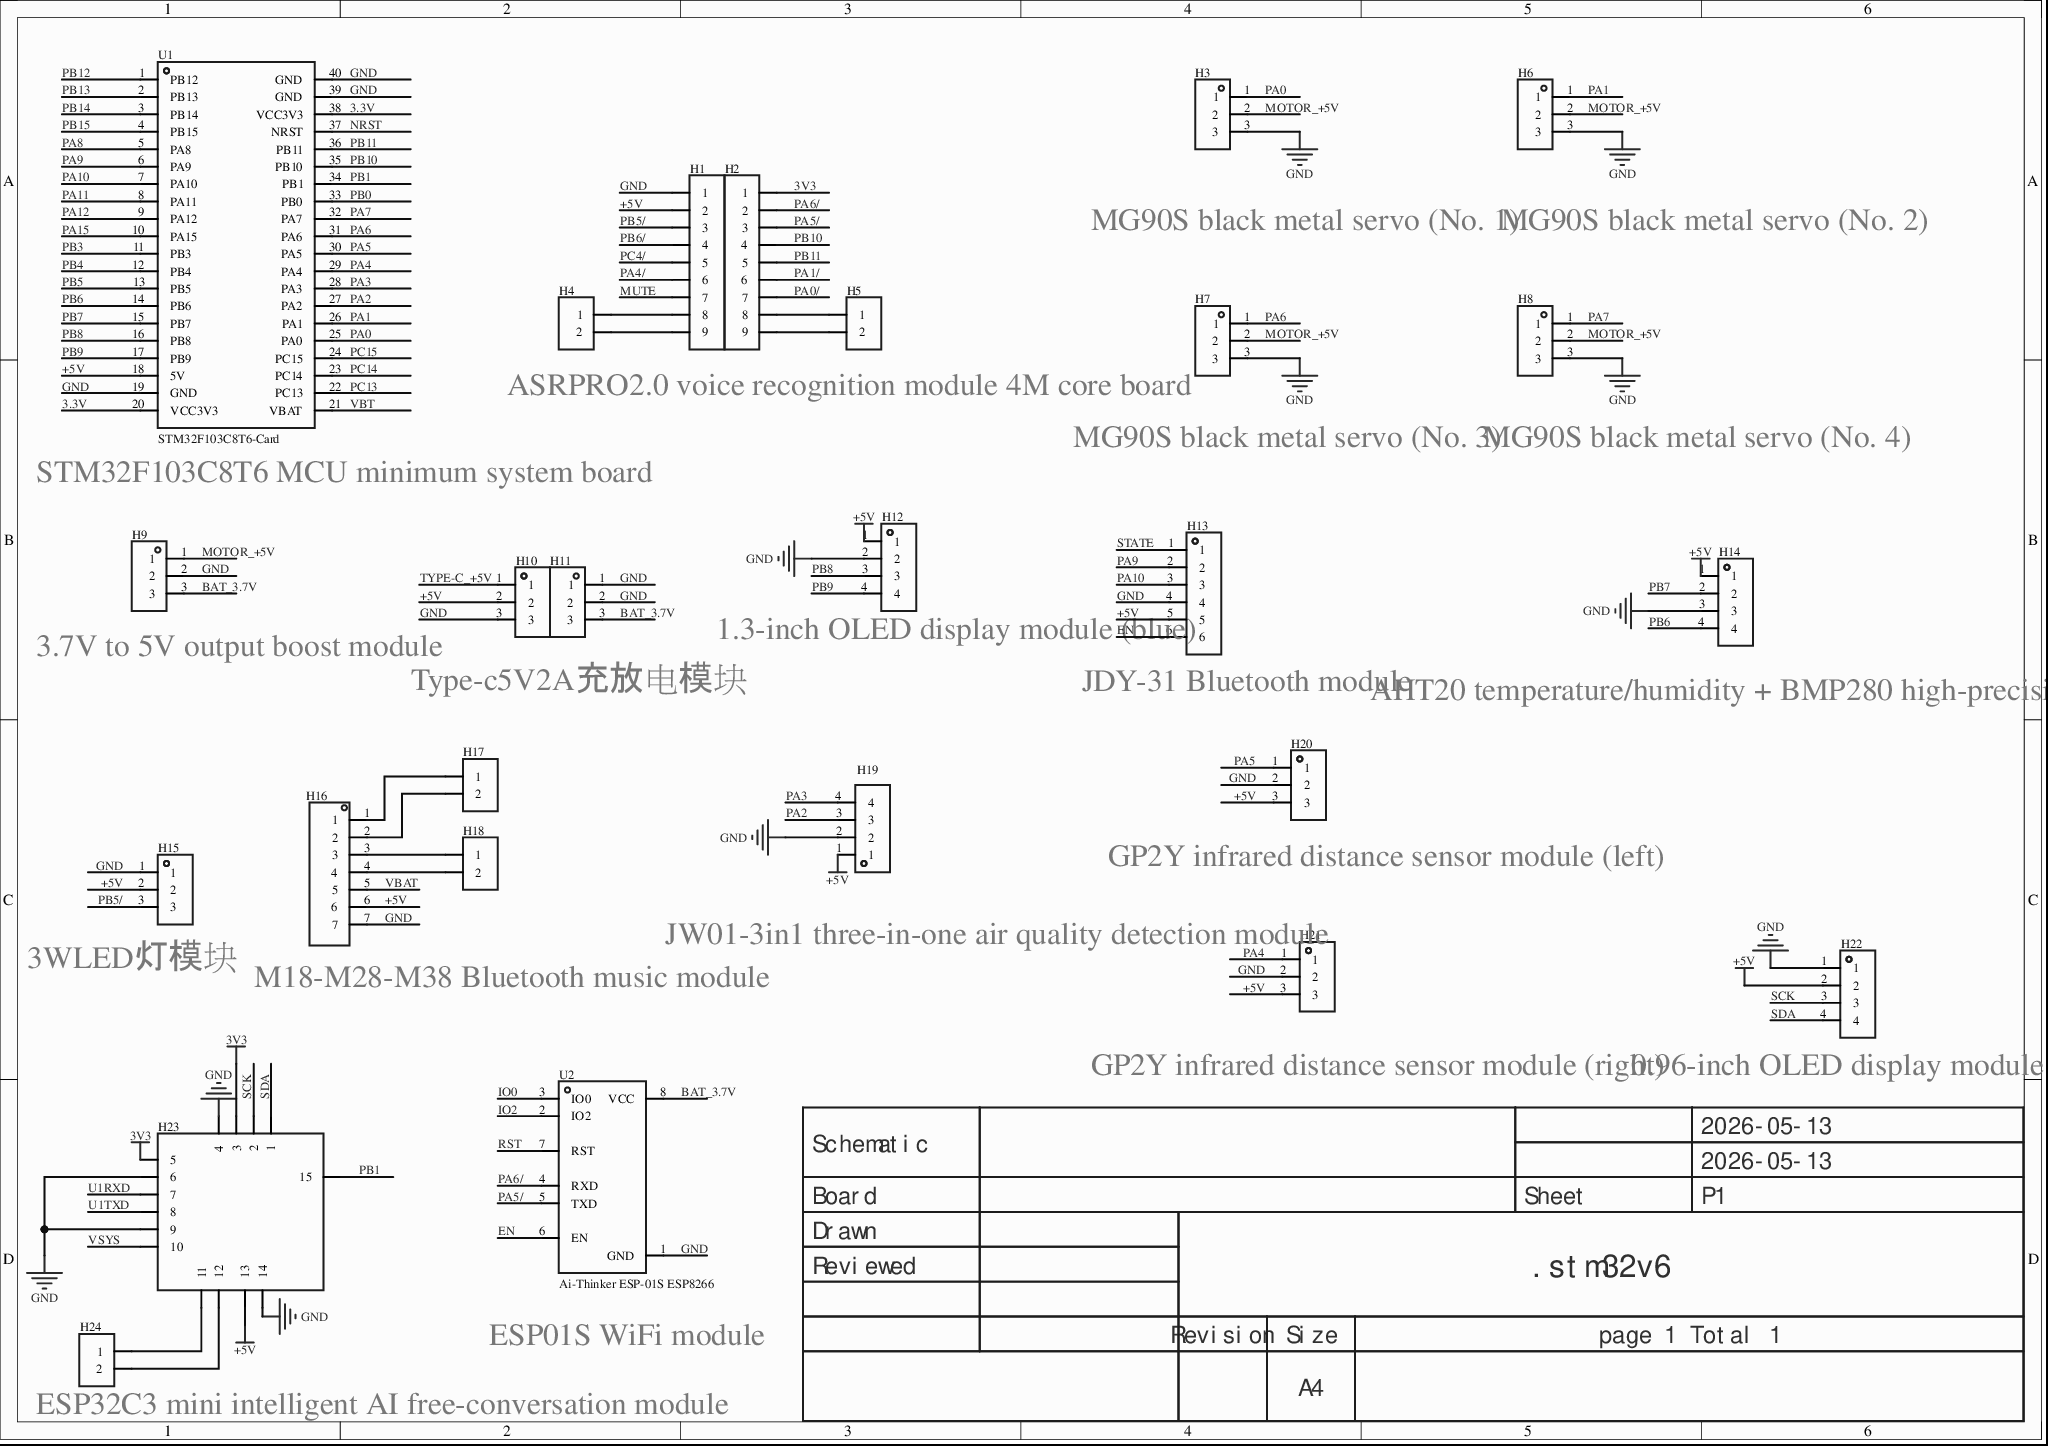
[diagram p0: MISC49865-3.schdoc]
# Altium project MISC49865-2.PrjPcb
1 sheet, 26 parts. Net scope: global (net labels, ports and power ports of the same name join across sheets).
Board file: MISC49865.pcbdoc

## Sheet MISC49865-3.schdoc
size 297 x 209 mm; Version: V1.0; @Project Name: MISC49865; @Page Count: 1; @Update Date: 2026-05-13; @Create Date: 2026-05-13; @Schematic Name: MISC49865; @Page No: 1; @Create Time: 23:22:16; @Update Time: 17:32:40; @Board Name: MISC49865

### Parts
H1  (no value)  [HDR-TH_9P-P2.54-V-F-1]
H2  (no value)  [HDR-TH_9P-P2.54-V-F-1]
H3  (no value)  [HDR-TH_3P-P2.54-V-F]
H4  (no value)  [HDR-TH_2P-P2.54-V-F]
H5  (no value)  [HDR-TH_2P-P2.54-V-F]
H6  (no value)  [HDR-TH_3P-P2.54-V-F]
H7  (no value)  [HDR-TH_3P-P2.54-V-F]
H8  (no value)  [HDR-TH_3P-P2.54-V-F]
H9  (no value)  [HDR-TH_3P-P2.54-V-F]
H10  (no value)  [HDR-TH_3P-P2.54-V-F]
H11  (no value)  [HDR-TH_3P-P2.54-V-F]
H12  (no value)  [HDR-TH_4P-P2.54-V-F]
H13  (no value)  [HDR-TH_6P-P2.54-V-F]
H14  (no value)  [HDR-TH_4P-P2.54-V-F]
H15  (no value)  [HDR-TH_3P-P2.54-V-F]
H16  (no value)  [HDR-TH_7P-P2.54-V-F]
H17  (no value)  [HDR-TH_2P-P2.54-V-F]
H18  (no value)  [HDR-TH_2P-P2.54-V-F]
H19  (no value)  [HDR-TH_4P-P2.54-V-F]
H20  (no value)  [HDR-TH_3P-P2.54-V-F]
H21  (no value)  [HDR-TH_3P-P2.54-V-F]
H22  (no value)  [HDR-TH_4P-P2.54-V-F]
H23  (no value)  [ESP32C3MINI]
H24  (no value)  [HDR-TH_2P-P2.54-V-F]
U1  STM32F103C8T6-Card  [CONN-TH_L53.3-W22.9_STM32F103C8T6-CARD]
U2  Ai-Thinker ESP-01S ESP8266  [WIFIM-TH_8P-L24.7-W14.4-P2.54]

### Nets
3V3: H2.1 H23.3 H23.5
+5V: H1.2 H10.2 H12.1 H13.5 H14.1 H15.2 H16.6 H19.1 H20.3 H21.3 H22.2 H23.13 U1.18(5V)
GND: H1.1 H3.3 H6.3 H7.3 H8.3 H9.2 H10.3 H11.1 H11.2 H12.2 H13.4 H14.3 H15.1 H16.7 H19.2 H20.2 H21.2 H22.1 H23.4 H23.6 H23.9 H23.14 U1.19(GND) U1.39(GND) U1.40(GND) U2.1(GND)
3.3V: U1.20(VCC3V3) U1.38(VCC3V3)
BAT_3.7V: H9.3 H11.3 U2.8(VCC)
EN: H13.6 U2.6(EN)
IO0: U2.3(IO0)
IO2: U2.2(IO2)
MOTOR_+5V: H3.2 H6.2 H7.2 H8.2 H9.1
MUTE: H1.7
NRST: U1.37(NRST)
PA0: H3.1 U1.25(PA0)
PA0/: H2.7
PA1: H6.1 U1.26(PA1)
PA1/: H2.6
PA2: H19.3 U1.27(PA2)
PA3: H19.4 U1.28(PA3)
PA4: H21.1 U1.29(PA4)
PA4/: H1.6
PA5: H20.1 U1.30(PA5)
PA5/: H2.3 U2.5(TXD)
PA6: H7.1 U1.31(PA6)
PA6/: H2.2 U2.4(RXD)
PA7: H8.1 U1.32(PA7)
PA8: U1.5(PA8)
PA9: H13.2 U1.6(PA9)
PA10: H13.3 U1.7(PA10)
PA11: U1.8(PA11)
PA12: U1.9(PA12)
PA15: U1.10(PA15)
PB0: U1.33(PB0)
PB1: H23.15 U1.34(PB1)
PB3: U1.11(PB3)
PB4: U1.12(PB4)
PB5: U1.13(PB5)
PB5/: H1.3 H15.3
PB6: H14.4 U1.14(PB6)
PB6/: H1.4
PB7: H14.2 U1.15(PB7)
PB8: H12.3 U1.16(PB8)
PB9: H12.4 U1.17(PB9)
PB10: H2.4 U1.35(PB10)
PB11: H2.5 U1.36(PB11)
PB12: U1.1(PB12)
PB13: U1.2(PB13)
PB14: U1.3(PB14)
PB15: U1.4(PB15)
PC4/: H1.5
PC13: U1.22(PC13)
PC14: U1.23(PC14)
PC15: U1.24(PC15)
RST: U2.7(RST)
SCK: H22.3 H23.2
SDA: H22.4 H23.1
STATE: H13.1
TYPE-C_+5V: H10.1
U1RXD: H23.7
U1TXD: H23.8
VBAT: H16.5
VBT: U1.21(VBAT)
VSYS: H23.10
NetH1_8: H1.8 H4.1
NetH1_9: H1.9 H4.2
NetH2_8: H2.8 H5.1
NetH2_9: H2.9 H5.2
NetH16_1: H16.1 H17.1
NetH16_2: H16.2 H17.2
NetH16_3: H16.3 H18.1
NetH16_4: H16.4 H18.2
NetH23_11: H23.11 H24.1
NetH23_12: H23.12 H24.2

### Notes on the sheet
- MG90S black metal servo (No. 1)
- MG90S black metal servo (No. 2)
- (near H7) ASRPRO2.0 voice recognition module 4M core board
- STM32F103C8T6 MCU minimum system board
- MG90S black metal servo (No. 3)
- (near H8) MG90S black metal servo (No. 4)
- (near H10) 3.7V to 5V output boost module
- Type-c5V2A充放电模块
- (near H13) 1.3-inch OLED display module (blue)
- (near H13) JDY-31 Bluetooth module
- (near H14) AHT20 temperature/humidity + BMP280 high-precision barometric pressure module
- (near H20) GP2Y infrared distance sensor module (left)
- (near H21) JW01-3in1 three-in-one air quality detection module
- (near H15) 3WLED灯模块
- (near H16) M18-M28-M38 Bluetooth music module
- GP2Y infrared distance sensor module (right)
- (near H22) 0.96-inch OLED display module (black)
- (near U2) ESP01S WiFi module
- (near H24) ESP32C3 mini intelligent AI free-conversation module
- 2026-05-13
- Schematic
- Board
- Sheet
- P1
- Drawn
- Reviewed
- .stm32v6
- Revision
- Size
- A4
- page 1 Total 1

### Library data of the parts
H1 H2 = HDR-F_2.54_1x9P: Symbol: Header-Female-2.54_1x9; AddInBom: yes; ModelId: 3a7016416d904017ac5ead6cc0f14e9c0819f05c4eef4c71ace90d822a990e87; ModelName: HDR-TH_9P-P2.54-F-LI-1X9P; ModelTransform: 915.746,94.488,0,0,0,0,0,0,-125.984; Device: HDR-F_2.54_1x9P; ConvertToPcb: yes; FootprintName: HDR-TH_9P-P2.54-V-F-1; SupplierPart: C39576; Supplier Footprint: 插件
H3 H6-H11 H15 H20 H21 = HDR-F_2.54_1x3P: Symbol: PM254V-11-03-H85; 3D Model: f3b3cc5aae9641bf9e56fc160cef875b; 3D Model Transform: 299.9994,100,0,0,0,0,0,0,-118.11; ConvertToPcb: yes; ModelName: HDR2.54-F-LI-1X3P; Device: HDR-F_2.54_1x3P; Supplier Part: C541850; Supplier Footprint: 插件; AddInBom: yes; FootprintName: HDR-TH_3P-P2.54-V-F
H4 H5 H17 H18 = HDR-F_2.54_1x2P: Symbol: Header-Female-2.54_1x2; ConvertToPcb: yes; ModelId: a9450ef445564560a104363b9aacde4e; ModelName: HDR-TH_2P-P2.54-F-LI-1X2P; ModelTransform: 215.7476,98.425,0,0,0,0,0,0,-129.921; Device: HDR-F_2.54_1x2P; AddInBom: yes; SupplierPart: C49661; Supplier Footprint: 插件; FootprintName: HDR-TH_2P-P2.54-V-F
H12 H14 H19 H22 = HDR-F_2.54_1x4P: Symbol: 2.54-1*4P female; ConvertToPcb: yes; ModelId: d187812051054f85879fcaa51a310d8e0819f05c4eef4c71ace90d822a990e87; ModelTransform: 419.6842,98.464,0,0,0,0,0,0,-118.11; Device: HDR-F_2.54_1x4P; AddInBom: yes; SupplierPart: C2718488; Supplier Footprint: 插件; FootprintName: HDR-TH_4P-P2.54-V-F; ModelName: HDR-TH_4P-P2.54-V-F
H13 = HDR-F_2.54_1x6P: Symbol: Header-Female-2.54_1x6; ConvertToPcb: yes; ModelId: 0f5bcf94dcda47d085f24cdca1696fe9; ModelTransform: 619.684,94.488,0,0,0,0,0,0,-125.984; Device: HDR-F_2.54_1x6P; AddInBom: yes; SupplierPart: C40877; Supplier Footprint: 插件; FootprintName: HDR-TH_6P-P2.54-V-F; ModelName: HDR-TH_6P-P2.54-V-F
H16 = HDR-F_2.54_1x7P: Symbol: 220S-1*7P H=8.5MM Ytype Gold-plated; ConvertToPcb: yes; ModelId: 4c31987253bc43b9b52c17be2a6d3f910819f05c4eef4c71ace90d822a990e87; ModelName: HDR-TH_7P-P2.54-F-LI-1X7P; ModelTransform: 715.7466,94.488,0,0,0,0,0,0,-118.11; Device: HDR-F_2.54_1x7P; AddInBom: yes; SupplierPart: C124418; Supplier Footprint: 插件; FootprintName: HDR-TH_7P-P2.54-V-F
H23 = HDR-F_2.54_2x8: Symbol: HDR-F-2.54_2x8; ConvertToPcb: yes; ModelId: f6b5f7d40ec74b809fbaeebc5002f6e00819f05c4eef4c71ace90d822a990e87; ModelName: HDR2.54-F-LI-2X8P; ModelTransform: 799.99844,200,0,0,0,0,0,0,-118.11; Device: HDR-F_2.54_2x8; AddInBom: yes; SupplierPart: C30734; Supplier Footprint: 插件; FootprintName: ESP32C3MINI
H24 = HDR-F_2.54_1x2P: Symbol: Header-Female-2.54_1x2; 3D Model: a9450ef445564560a104363b9aacde4e; 3D Model Transform: 215.7476,98.425,0,0,0,0,0,0,-129.921; ConvertToPcb: yes; ModelName: HDR-TH_2P-P2.54-F-LI-1X2P; Device: HDR-F_2.54_1x2P; Supplier Part: C49661; Supplier Footprint: 插件; AddInBom: yes; FootprintName: HDR-TH_2P-P2.54-V-F
U1 = STM32F103C8T6-Card: AddInBom: yes; Symbol: STM32F103C8T6-CARD; Device: STM32F103C8T6-Card; LCSC Part Name: STM32F103C8T6-Card; SupplierPart: C9900077949; ManufacturerPart: STM32F103C8T6-Card; Supplier Footprint: 插件; Supplier: LCSC; ConvertToPcb: yes; FootprintName: CONN-TH_L53.3-W22.9_STM32F103C8T6-CARD
U2 = Ai-Thinker ESP-01S ESP8266: Manufacturer: Ai-Thinker(安信可); AddInBom: yes; ModelId: 9453774c1eaa4779b246df5901e962460819f05c4eef4c71ace90d822a990e87; ModelName: WIFIM-TH_8P-L24.7-W14.4-H2.8-P2.54; ModelTransform: 972.43904,566.928,0,0,0,0,377.167,-3.936,-118.11; Symbol: AI-THINKER ESP-01S ESP8266; Device: Ai-Thinker ESP-01S ESP8266; LCSC Part Name: Ai-Thinker ESP-01S ESP8266; SupplierPart: C17606792; ManufacturerPart: Ai-Thinker ESP-01S ESP8266; Supplier Footprint: -; JLCPCB Part Class: Extended Part; Datasheet: https://item.szlcsc.com/datasheet/Ai-Thinker%2520ESP-01S%2520ESP8266/18736031.html; Supplier: LCSC; ConvertToPcb: yes; FootprintName: WIFIM-TH_8P-L24.7-W14.4-P2.54